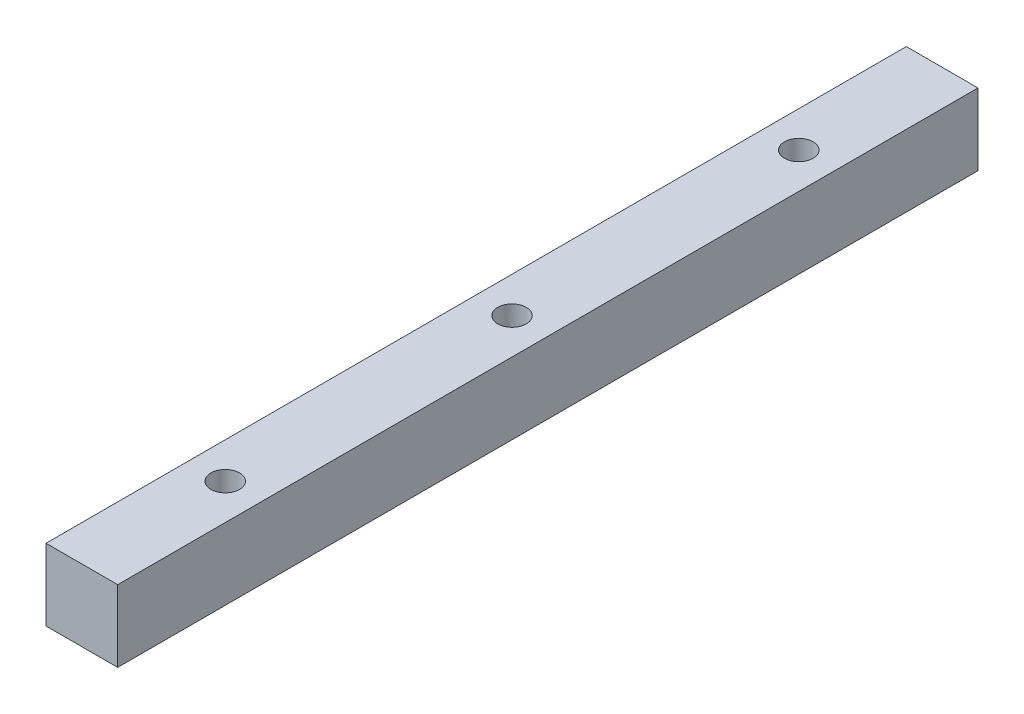
from build123d import *

# Parameters (mm, degrees)
SKETCH_1_W             = 15
SKETCH_1_H             = 15
EXTRUDE_1_DEPTH        = 90
SKETCH_2_R             = 3
CUT_EXTRUDE_1_DEPTH    = 4.5
SKETCH_3_R             = 2
CUT_EXTRUDE_2_DEPTH    = 92.549167118
PATTERN_LINEAR_1_COUNT = 4
PATTERN_LINEAR_1_PITCH = 60


with BuildPart() as part:
    # 草图1 → 凸台-拉伸1 (new, symmetric)
    with BuildSketch(Plane.XY):
        Rectangle(SKETCH_1_W, SKETCH_1_H)
    extrude(amount=EXTRUDE_1_DEPTH, both=True)

    # 草图2 → 切除-拉伸1 (cut)
    with BuildSketch(Plane(origin=(0, 7.5, 0), x_dir=(1, 0, 0), z_dir=(0, 1, 0))):
        with Locations(Location((0, -60, 0), (0, 0, 270))):
            Circle(SKETCH_2_R)
    cut_extrude_1 = extrude(amount=-CUT_EXTRUDE_1_DEPTH, mode=Mode.SUBTRACT)

    # 草图3 → 切除-拉伸2 (cut, through all)
    with BuildSketch(Plane(origin=(0, 7.5, 0), x_dir=(1, 0, 0), z_dir=(0, 1, 0))):
        with Locations(Location((0, -60, 0), (0, 0, 270))):
            Circle(SKETCH_3_R)
    cut_extrude_2 = extrude(amount=-CUT_EXTRUDE_2_DEPTH, mode=Mode.SUBTRACT)

    # 阵列(线性)1: 切除-拉伸1, 切除-拉伸2 ×4
    with Locations(*[(0, 0, -i * PATTERN_LINEAR_1_PITCH) for i in range(1, PATTERN_LINEAR_1_COUNT)]):
        add(cut_extrude_1, mode=Mode.SUBTRACT)
        add(cut_extrude_2, mode=Mode.SUBTRACT)


solid = part.part
